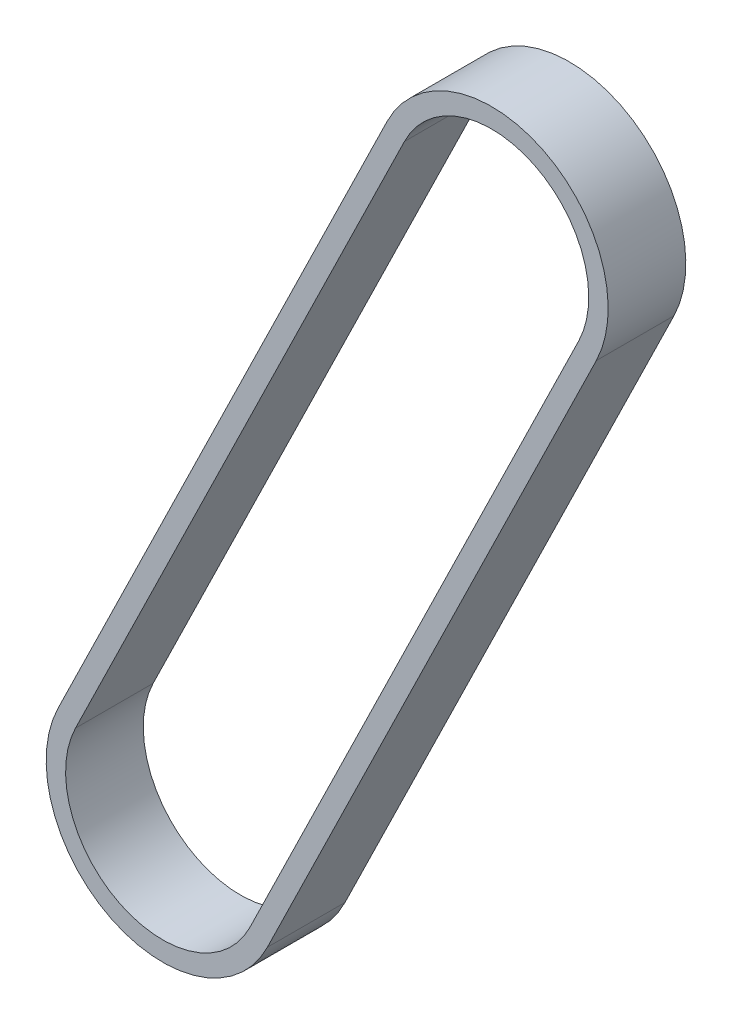
from build123d import *

# Parameters (mm, degrees)
EXTRUDE_1_DEPTH = 40


with BuildPart() as part:
    # 草图1 → 凸台-拉伸1 (new, symmetric)
    with BuildSketch(Plane.XY):
        with BuildLine():
            Line((878.652807565, 894.525207523), (539.795222723, 201.743243487))
            ThreePointArc((539.795222723, 201.743243487), (594.86543093, 41.221369064), (755.387305352, 96.291577272))
            Line((755.387305352, 96.291577272), (1094.244890195, 789.073541309))
            ThreePointArc((1094.244890195, 789.073541309), (1039.174681987, 949.595415731), (878.652807565, 894.525207523))
        make_face()
        with BuildLine():
            Line((896.618814451, 885.737568672), (557.761229608, 192.955604635))
            ThreePointArc((557.761229608, 192.955604635), (603.653069781, 59.18737595), (737.421298466, 105.079216123))
            Line((737.421298466, 105.079216123), (1076.278883309, 797.86118016))
            ThreePointArc((1076.278883309, 797.86118016), (1030.387043136, 931.629408845), (896.618814451, 885.737568672))
        make_face(mode=Mode.SUBTRACT)
    extrude(amount=EXTRUDE_1_DEPTH, both=True)


solid = part.part
